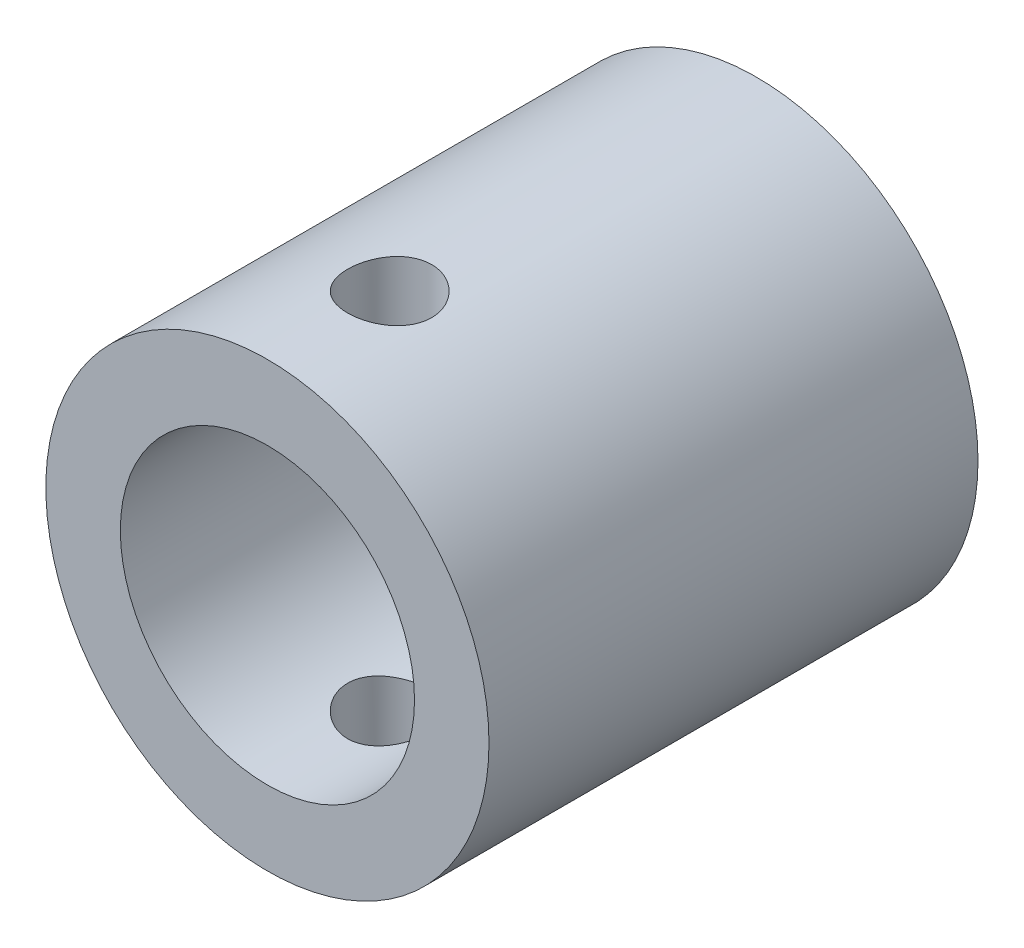
SolidWorks part; units mm, degrees
material "40r"
ref_plane "Front Plane" through (0, 0, 0) normal (0, 0, 1) x (1, 0, 0)
ref_plane "Top Plane" through (0, 0, 0) normal (0, 1, 0) x (1, 0, 0)
ref_plane "Right Plane" through (0, 0, 0) normal (1, 0, 0) x (0, 0, -1)
sketch "Sketch1" plane through (0, 0, 0) normal (0, 0, 1) x (1, 0, 0)
  circle A0 centre (0, 0) radius 58
  circle A1 centre (0, 0) radius 24
  dimension "D1" = 116
  dimension "D2" = 48
extrude "Boss-Extrude1" add sketch "Sketch1" along normal blind 128
sketch "Sketch2" plane through (0, 0, 128) normal (0, 0, 1) x (1, 0, 0)
  circle A0 centre (0, 0) radius 38
  dimension "D1" = 76
extrude "Cut-Extrude1" cut sketch "Sketch2" against normal blind 102
sketch "Sketch3" plane through (0, 0, 0) normal (0, 1, 0) x (1, 0, 0)
  line L1 (-58, -128) -> (58, -128) construction
  circle A0 centre (0, -96) radius 11
  dimension "D1" = 22
  dimension "D2" = 32
extrude "Cut-Extrude2" cut sketch "Sketch3" against normal through all both and the other way through all
sketch "Sketch6" plane through (0, 0, 128) normal (0, 0, 1) x (1, 0, 0)
  circle A0 centre (0, 0) radius 38.5
  dimension "D1" = 77
extrude "Cut-Extrude3" cut sketch "Sketch6" against normal blind 68
cosmetic thread "Cosmetic thread2" parameters "D2"=80
sketch "Sketch7" plane through (0, 0, 60) normal (0, 0, 1) x (1, 0, 0)
  circle A0 centre (0, 0) radius 40
  dimension "D1" = 80
extrude "Cut-Extrude4" cut sketch "Sketch7" along normal blind 4
